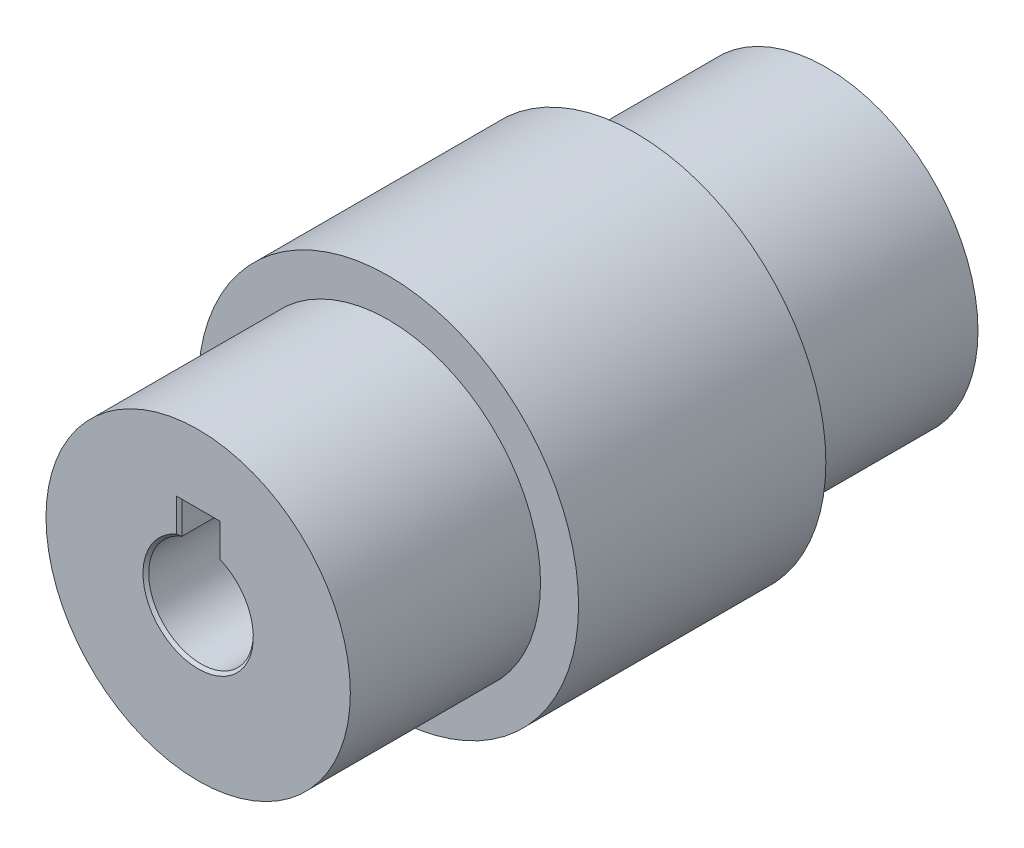
SolidWorks part; units mm, degrees
ref_plane "前视" through (0, 0, 0) normal (0, 0, 1) x (1, 0, 0)
ref_plane "上视" through (0, 0, 0) normal (0, 1, 0) x (1, 0, 0)
ref_plane "右视" through (0, 0, 0) normal (1, 0, 0) x (0, 0, -1)
sketch "草图1" plane through (0, 0, 0) normal (0, 0, 1) x (0, -1, 0)
  circle A0 centre (0, 0) radius 16
extrude "拉伸1" add sketch "草图1" along normal blind 20
sketch "草图2" plane through (0, 0, 20) normal (0, 0, 1) x (0, 1, 0)
  circle A0 centre (0, 0) radius 20
extrude "拉伸2" add sketch "草图2" along normal blind 26
sketch "草图3" plane through (0, 0, 46) normal (0, 0, 1) x (0, 1, 0)
  circle A0 centre (0, 0) radius 16
extrude "拉伸3" add sketch "草图3" along normal blind 20
sketch "草图4" plane through (0, 0, 0) normal (0, 0, -1) x (-1, 0, 0)
  circle A0 centre (0, 0) radius 9.5
  dimension "D1" = 19
extrude "切除-拉伸1" cut sketch "草图4" against normal blind 27
sketch "草图5" plane through (0, 0, 66) normal (0, 0, 1) x (1, 0, 0)
  circle A0 centre (0, 0) radius 5.5
  dimension "D1" = 11
extrude "切除-拉伸2" cut sketch "草图5" against normal blind 27
sketch "草图6" plane through (0, 0, 39) normal (0, 0, 1) x (1, 0, 0)
  circle A0 centre (0, 0) radius 10
extrude "切除-拉伸3" cut sketch "草图6" against normal blind 12
sketch "草图7" plane through (0, 0, 0) normal (0, 0, -1) x (-1, 0, 0)
  line L0 (0, 0) -> (0, 16) construction
  line L1 (-3, 12) -> (-3, 9.0139)
  line L2 (-3, 12) -> (3, 12)
  line L3 (3, 12) -> (3, 9.0139)
  circle A0 centre (0, 0) radius 16 construction
  circle A1 centre (0, 0) radius 9.5 construction
  arc A2 (3, 9.0139) -> (-3, 9.0139) centre (0, 0) ccw
  dimension "D1" = 6
  dimension "D2" = 3
  dimension "D3" = 12
extrude "切除-拉伸4" cut sketch "草图7" against normal blind 27
sketch "草图8" plane through (0, 0, 66) normal (0, 0, 1) x (1, 0, 0)
  line L0 (0, 16) -> (0, 0) construction
  line L1 (-2, 8.5) -> (-2, 5.1235)
  line L2 (-2, 8.5) -> (2, 8.5)
  line L3 (2, 8.5) -> (2, 5.1235)
  circle A0 centre (0, 0) radius 16 construction
  circle A1 centre (0, 0) radius 5.5 construction
  arc A2 (2, 5.1235) -> (-2, 5.1235) centre (0, 0) ccw
  dimension "D1" = 4
  dimension "D2" = 2
  dimension "D3" = 8.5
extrude "切除-拉伸5" cut sketch "草图8" against normal blind 27
chamfer "倒角1" distance 0.3 angle 45 8 edges at (-3, 10.5069, 0) (0, 12, 0) (3, 10.5069, 0) (0, -9.5, 0) (2, 6.8117, 66) (0, 8.5, 66) (-2, 6.8117, 66) (0, -5.5, 66)
